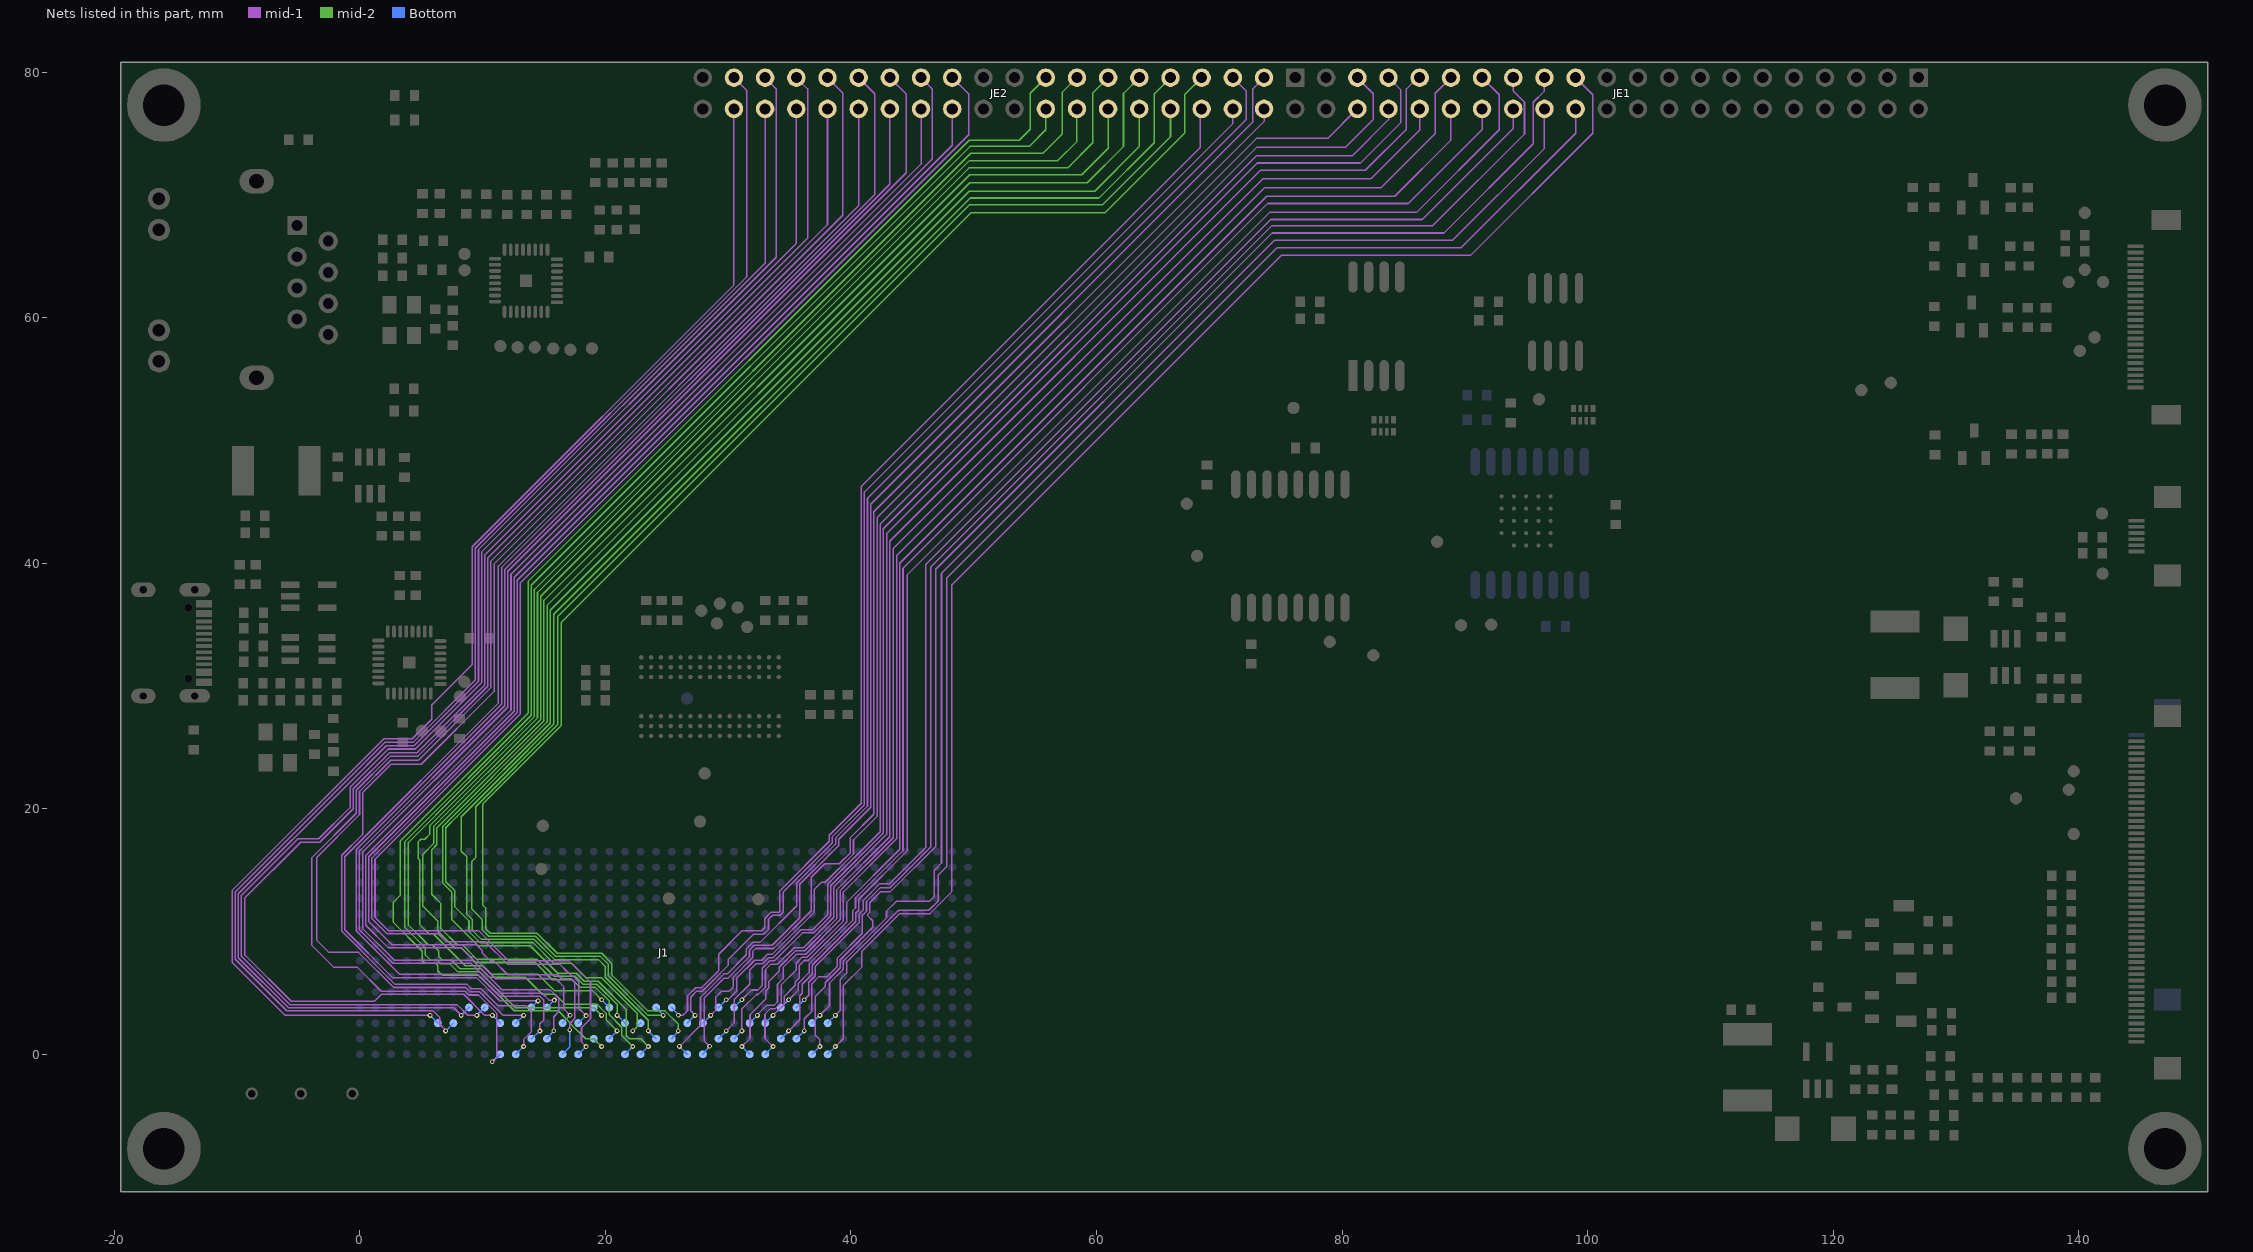
[diagram p0: the nets of this part, all layers, seen from the top]
# Altium PCB MISC105414.PcbDoc (part 5 of 11)
Units mm, origin at the board's own origin, x right, y up, seen from the top; angles counter-clockwise.
Board outline 170 x 92 mm, 6 copper layers (Top, GND, mid-1, mid-2, mid-3, Bottom), stack 1.231 mm thick; 238 components, 304 nets, 1456 pads, 1258 vias.
Unrouted connection lines stored in the file: 57.

## Via types
v1: diameter 0.4, hole 0.2, Top to Bottom, tented top, 618 vias
v2: diameter 0.5, hole 0.3, Top to Bottom, tented top, 522 vias
v3: diameter 0.5, hole 0.3, Top to Bottom, 41 vias
v4: diameter 1, hole 0.5, Top to Bottom, tented top, 36 vias
v5: diameter 0.7, hole 0.4, Top to Bottom, tented top, 34 vias
v6: diameter 1.3, hole 1.3, Top to Bottom, tented top, 3 vias
v7: diameter 4, hole 4, Top to Bottom, tented top, 2 vias
v8: diameter 3.3, hole 3.3, Top to Bottom, tented top, 2 vias

## Nets (pads, with @x,y where several pads share a name; then routed paths per layer and width w, separated by ;. In a path a pad name is that pad's centre, name@x,y a point inside that pad or via, vN(x,y) a via of type N, cw(c..) or ccw(c..) an arc to the next point about the centre after c; other vN are vias at no path point) (continued)
EXT_IO16: J1.Y10 JE1.23 | length 116.4
  mid-1 w0.127: v1(38.735,0.635) 39.37,1.27 39.37,5.594 40.896,7.12 40.896,8.39 43.97,11.465 46.438,11.465 48.2,13.227 48.2,38.2 75.1,65.1 90.5,65.1 100.421,75.021 100.421,78.159 JE1.23@99.03,79.55
  Bottom w0.127: J1.Y10@38.1,0 v1(38.735,0.635)
EXT_IO17: J1.A10 JE1.24 | length 109.9
  mid-1 w0.127: v1(38.735,3.175) 39.115,3.555 39.115,6.095 39.642,6.622 39.642,7.495 43.85,11.703 43.883,11.703 43.89,11.709 43.902,11.709 43.906,11.713 43.918,11.713 43.923,11.718 43.948,11.718 43.959,11.729 46.343,11.729 47.104,12.489 47.104,14.598 47.8,15.294 47.8,38.8 74.7,65.7 89.7,65.7 99.03,75.03 JE1.24@99.03,77.01
  Bottom w0.127: J1.A10@38.1,2.54 v1(38.735,3.175)
EXT_IO18: J1.Y11 JE1.25 | length 113.6
  mid-1 w0.127: v1(37.465,0.635) 37.465,1.195 37.102,1.558 37.102,4.717 37.913,5.528 37.913,5.82 39.134,7.04 39.134,7.707 41.771,10.345 41.771,10.879 41.353,11.297 41.353,11.387 41.522,11.556 41.522,12.343 42.429,13.251 43.217,13.251 46.9,16.934 46.9,39.5 74.3,66.9 88.3,66.9 95.576,74.176 95.576,77.556 96.49,78.469 JE1.25@96.49,79.55
  Bottom w0.127: J1.Y11@36.83,0 v1(37.465,0.635)
EXT_IO19: J1.A11 JE1.26 | length 109.3
  mid-1 w0.127: v1(37.465,3.175) 38.252,3.962 38.252,5.799 39.388,6.935 39.388,7.6 42.897,11.11 42.897,11.662 43.687,12.451 46.376,12.451 46.8,12.875 46.8,15 47.375,15.575 47.375,39.175 74.5,66.3 89,66.3 96.49,73.79 JE1.26@96.49,77.01
  Bottom w0.127: J1.A11@36.83,2.54 v1(37.465,3.175)
EXT_IO20: J1.Z12 JE1.27 | length 111.7
  mid-1 w0.127: v1(36.195,1.905) 36.195,2.885 36.821,3.511 36.821,5.754 37.399,6.332 38.066,6.332 38.868,7.134 38.868,7.801 40.918,9.851 40.918,11.312 41.267,11.66 41.267,12.448 42.369,13.55 43.157,13.55 46.5,16.893 46.5,39.7 74.3,67.5 87.4,67.5 94.863,74.963 94.863,77.556 93.95,78.469 JE1.27@93.95,79.55
  Bottom w0.127: J1.Z12@35.56,1.27 v1(36.195,1.905)
EXT_IO21: J1.B12 JE1.28 | length 105.1
  mid-1 w0.127: v1(36.195,4.445) 36.567,4.817 36.567,5.863 37.097,6.393 37.097,7.142 40.663,10.708 40.663,11.416 41.013,11.765 41.013,12.553 42.335,13.875 43.123,13.875 46.1,16.852 46.1,39.9 74.2,68 86.537,68 93.95,75.413 JE1.28@93.95,77.01
  Bottom w0.127: J1.B12@35.56,3.81 v1(36.195,4.445)
EXT_IO22: J1.Z13 JE1.29 | length 110.1
  mid-1 w0.127: v1(34.925,1.905) 35.832,2.812 35.832,4.77 36.029,4.967 36.029,5.712 36.842,6.526 36.842,7.246 40.396,10.8 40.396,11.508 40.627,11.739 40.627,12.628 44.6,16.601 44.6,39.073 74.127,68.6 86.1,68.6 92.8,75.3 92.8,78.16 JE1.29@91.41,79.55
  Bottom w0.127: J1.Z13@34.29,1.27 v1(34.925,1.905)
EXT_IO23: J1.B13 JE1.30 | length 103.6
  mid-1 w0.127: v1(34.925,4.445) 35.721,5.241 35.721,5.79 36.588,6.658 36.588,7.352 40.134,10.897 40.134,11.68 40.371,11.917 40.371,12.731 44.238,16.598 44.238,39.6 73.938,69.3 85.4,69.3 91.41,75.31 JE1.30@91.41,77.01
  Bottom w0.127: J1.B13@34.29,3.81 v1(34.925,4.445)
EXT_IO24: J1.Y14 JE1.31 | length 109.2
  mid-1 w0.127: v1(33.655,0.635) 33,1.29 33,3.275 33.45,3.725 33.846,3.725 34.308,4.187 34.308,5.642 35.538,6.872 35.538,7.416 36.019,7.897 36.415,7.897 39.384,10.865 39.384,13.228 43.714,17.558 43.714,40.6 73.714,70.6 83.2,70.6 87.6,75 87.6,78.28 JE1.31@88.87,79.55
  Bottom w0.127: J1.Y14@33.02,0 v1(33.655,0.635)
EXT_IO25: J1.A14 JE1.32 | length 103.9
  mid-1 w0.127: v1(33.655,3.175) 34.562,4.082 34.562,4.717 35.467,5.622 35.467,5.895 35.792,6.22 35.792,7.223 36.206,7.638 36.516,7.638 39.641,10.764 39.641,12.361 43.979,16.698 43.979,40 73.879,69.9 84.3,69.9 88.87,74.47 JE1.32@88.87,77.01
  Bottom w0.127: J1.A14@33.02,2.54 v1(33.655,3.175)
EXT_IO26: J1.Y15 JE1.33 | length 108.2
  mid-1 w0.127: v1(31.115,0.635) 31.775,1.295 31.775,3.225 33.05,4.5 33.05,5.135 33.292,5.377 33.292,5.916 34.15,6.775 34.15,7.097 35.485,8.432 36.232,8.432 38.857,11.057 38.857,13.42 43.159,17.722 43.159,41.8 73.359,72 81.9,72 85.25,75.35 85.25,78.634 86.167,79.55 JE1.33@86.33,79.55
  Bottom w0.127: v1(31.115,0.635) J1.Y15@31.75,0
EXT_IO27: J1.A15 JE1.34 | length 103
  mid-1 w0.127: v1(32.385,3.175) 32.385,3.235 33.129,3.979 33.741,3.979 34.018,4.257 34.018,5.712 34.475,6.169 34.475,7.063 35.566,8.154 36.313,8.154 39.116,10.957 39.116,13.319 43.439,17.642 43.439,41.2 73.539,71.3 82.35,71.3 86.33,75.28 JE1.34@86.33,77.01
  Bottom w0.127: J1.A15@31.75,2.54 v1(32.385,3.175)
EXT_IO28: J1.Z16 JE1.35 | length 107
  mid-1 w0.127: v1(31.115,1.905) 31.115,3.689 32.296,4.871 32.426,4.871 33.038,5.482 33.038,6.901 33.487,7.351 34.044,7.351 35.38,8.686 36.127,8.686 38.603,11.162 38.603,13.623 42.902,17.922 42.902,42.4 73.102,72.6 81.5,72.6 84.8,75.9 84.8,78.54 JE1.35@83.79,79.55
  Bottom w0.127: J1.Z16@30.48,1.27 v1(31.115,1.905)
EXT_IO29: J1.B16 JE1.36 | length 100.9
  mid-1 w0.127: v1(31.115,4.445) 31.908,5.238 32.422,5.238 32.784,5.599 32.784,7.007 33.382,7.606 33.761,7.606 36.044,9.888 36.97,9.888 38.349,11.267 38.349,13.738 42.638,18.027 42.638,42.8 73.038,73.2 80.85,73.2 83.79,76.14 JE1.36@83.79,77.01
  Bottom w0.127: J1.B16@30.48,3.81 v1(31.115,4.445)
EXT_IO30: J1.Z17 JE1.37 | length 106.2
  mid-1 w0.127: v1(29.845,1.905) 30.48,2.54 30.48,4.445 31.75,5.715 31.75,6.864 32.263,7.377 32.794,7.377 33.277,7.86 33.653,7.86 35.935,10.142 36.865,10.142 38.095,11.373 38.095,13.845 42.382,18.132 42.382,43.2 73.082,73.9 80.3,73.9 82.55,76.15 82.55,78.25 JE1.37@81.25,79.55
  Bottom w0.127: J1.Z17@29.21,1.27 v1(29.845,1.905)
EXT_IO31: J1.B17 JE1.38 | length 99
  mid-1 w0.127: v1(29.845,4.445) 29.99,4.445 30.683,5.138 30.683,6.188 32.162,7.668 32.726,7.668 33.191,8.132 33.566,8.132 37.022,11.589 37.022,13.433 37.609,14.021 37.912,14.021 40.208,16.317 40.208,17.458 42.127,19.377 42.127,43.697 73.031,74.6 78.84,74.6 JE1.38@81.25,77.01
  Bottom w0.127: J1.B17@29.21,3.81 v1(29.845,4.445)
EXT_IO32: J1.Y18 JE2.3 | length 99.9
  mid-1 w0.127: v1(28.483,0.651) 28.035,1.1 28.035,4.56 29.685,6.211 29.986,6.211 31.736,7.962 31.736,8.48 32.129,8.872 33.585,8.872 35.832,11.119 35.832,13.845 38.121,16.134 39.002,17.015 39.002,17.515 41.606,20.119 41.606,44.8 72.736,75.93 72.736,78.637 JE2.3@73.65,79.55
  Bottom w0.127: J1.Y18@27.94,0 v1(28.483,0.651)
EXT_IO33: J1.A18 JE2.4 | length 95.3
  mid-1 w0.127: v1(28.575,3.175) 29,3.6 29,4.675 29.443,5.118 30.055,5.118 30.396,5.459 30.396,6.262 31.99,7.857 31.99,8.374 32.234,8.618 33.693,8.618 36.768,11.694 36.768,14.422 37.858,15.512 39.043,15.512 39.954,16.422 39.954,17.654 41.861,19.561 41.861,44.2 73.65,75.989 JE2.4@73.65,77.01
  Bottom w0.127: J1.A18@27.94,2.54 v1(28.575,3.175)
EXT_IO34: J1.Y19 JE2.5 | length 99.9
  mid-1 w0.127: v1(26.027,0.643) 27.743,2.359 27.743,4.628 29.658,6.543 29.917,6.543 31.478,8.104 31.478,8.581 32.041,9.144 32.626,9.144 35.578,12.095 35.578,13.95 38.748,17.121 38.748,17.625 41.35,20.227 41.35,45.3 72.2,76.15 72.2,78.46 JE2.5@71.11,79.55
  Bottom w0.127: v1(26.027,0.643) J1.Y19@26.67,0
EXT_IO35: J1.A19 JE2.6 | length 94.3
  mid-1 w0.127: v1(27.305,3.175) 26.942,3.538 26.942,4.652 27.414,5.125 27.878,5.125 29.991,7.238 29.991,7.702 32.068,9.779 32.902,9.779 33.284,10.16 33.284,10.994 33.622,11.333 34.247,11.333 34.475,11.561 34.475,13.207 38.494,17.226 38.494,17.731 41.096,20.332 41.096,45.8 71.11,75.814 JE2.6@71.11,77.01
  Bottom w0.127: J1.A19@26.67,2.54 v1(27.305,3.175)
EXT_IO36: J1.Z20 JE2.7 | length 120.9
  mid-2 w0.127: v1(25.931,1.9) 25.931,2.459 24.859,3.53 23.464,3.53 20.503,6.492 20.503,7.422 19.7,8.225 16.075,8.225 14.434,9.866 10.609,9.866 10.239,10.236 10.239,11.92 10.006,12.153 10.006,20.382 16.4,26.776 16.4,35.18 49.77,68.55 60.7,68.55 67.2,75.05 67.2,78.18 JE2.7@68.57,79.55
  Bottom w0.127: J1.Z20@25.4,1.27 v1(25.931,1.9)
EXT_IO37: J1.B20 JE2.8 | length 94.1
  mid-1 w0.127: v1(25.949,3.179) 26.323,3.179 26.688,3.543 26.688,4.758 27.355,5.425 27.818,5.425 29.223,6.83 29.223,8.147 31.131,10.055 32.73,10.055 32.975,10.3 32.975,11.045 33.517,11.587 34.142,11.587 34.216,11.661 34.216,13.325 38.24,17.349 38.24,17.84 40.838,20.438 40.838,46.25 68.45,73.862 68.45,76.89 JE2.8@68.57,77.01
  Bottom w0.127: J1.B20@25.4,3.81 v1(25.949,3.179)
EXT_IO38: J1.Z21 JE2.9 | length 119.6
  mid-2 w0.127: 11.631,22.726 8.255,19.35 8.255,16.545 8.715,16.085 8.715,11.423 9.14,10.998 9.14,10.116 9.898,9.358 14.201,9.358 15.842,7.717 19.433,7.717 19.992,7.158 19.992,6.283 23.495,2.78 v1(23.495,1.905) ; 11.632,22.726 15.8,26.894 15.8,35.838 49.712,69.75 60.2,69.75 64.7,74.25 64.7,78.22 JE2.9@66.03,79.55
  Bottom w0.127: v1(23.495,1.905) J1.Z21@24.13,1.27
EXT_IO39: J1.B21 JE2.10 | length 116.2
  mid-2 w0.127: v1(24.709,3.167) 23.469,3.167 20.246,6.389 20.246,7.32 19.595,7.971 15.947,7.971 14.306,9.612 10.504,9.612 9.985,10.131 9.985,10.953 9.125,11.813 9.125,15.725 9.43,16.03 9.43,20.165 16.1,26.835 16.1,35.634 49.666,69.2 60.5,69.2 66.03,74.73 JE2.10@66.03,77.01
  Bottom w0.127: J1.B21@24.13,3.81 v1(24.709,3.167)
EXT_IO40: J1.Y22 JE2.11 | length 120.4
  mid-2 w0.127: v1(23.495,0.635) 22.874,1.256 21.963,1.256 21.705,1.514 21.705,3.657 19.409,5.954 18.27,5.954 17.617,6.607 16.118,6.607 13.875,8.85 9.613,8.85 7.484,10.979 7.484,13.213 6.74,13.958 6.74,18.554 15.247,27.061 15.247,36.566 49.682,71 59.25,71 62.2,73.95 62.2,78.26 JE2.11@63.49,79.55
  Bottom w0.127: J1.Y22@22.86,0 v1(23.495,0.635)
EXT_IO41: J1.A22 JE2.12 | length 116.1
  mid-2 w0.127: v1(22.225,1.905) 22.589,2.269 22.589,3.326 19.691,6.223 18.439,6.223 17.262,7.4 15.8,7.4 14.096,9.104 9.793,9.104 8.886,10.011 8.886,10.856 7.738,12.003 7.738,13.318 6.994,14.063 6.994,18.448 7.915,19.369 15.503,26.957 15.503,36.166 49.637,70.3 59.85,70.3 63.49,73.94 JE2.12@63.49,77.01
  Bottom w0.127: v1(22.225,1.905) J1.A22@22.86,2.54
EXT_IO42: J1.Y23 JE2.13 | length 119.5
  mid-2 w0.127: v1(22.225,0.635) 21.331,1.529 21.331,2.209 20.305,3.235 20.305,4.339 19.198,5.446 17.947,5.446 17.315,6.078 15.672,6.078 14.276,7.474 9.44,7.474 8.25,8.664 7.736,8.664 6.35,10.05 6.35,10.85 5.137,12.063 5.137,16.296 6.006,17.165 6.006,18.546 14.733,27.273 14.733,37.316 49.618,72.2 57.65,72.2 59.7,74.25 59.7,78.3 JE2.13@60.95,79.55
  Bottom w0.127: J1.Y23@21.59,0 v1(22.225,0.635)
EXT_IO43: J1.A23 JE2.14 | length 113.9
  mid-2 w0.127: v1(20.955,3.175) 20.955,4.048 19.303,5.7 18.165,5.7 17.511,6.353 15.822,6.353 14.447,7.728 9.545,7.728 8.356,8.918 7.932,8.918 6.604,10.246 6.604,12.291 5.85,13.045 5.85,16.649 6.261,17.06 6.261,18.437 14.988,27.163 14.988,36.966 49.672,71.65 58.8,71.65 60.95,73.8 JE2.14@60.95,77.01
  Bottom w0.127: v1(20.955,3.175) J1.A23@21.59,2.54
EXT_IO44: J1.Z24 JE2.15 | length 117.1
  mid-2 w0.127: v1(20.955,1.905) 20.051,2.809 20.051,3.324 19.309,4.067 16.709,4.067 15.878,4.898 14.85,4.898 13.477,6.271 10.562,6.271 9.867,6.966 8.159,6.966 7.475,7.65 6.725,7.65 6.438,7.937 6.438,8.384 5.904,8.918 5.56,8.918 3.95,10.527 3.95,17.25 8.361,21.661 14.214,27.514 14.214,37.866 49.749,73.4 55.65,73.4 57.2,74.95 57.2,78.34 JE2.15@58.41,79.55
  Bottom w0.127: J1.Z24@20.32,1.27 v1(20.955,1.905)
EXT_IO45: J1.B24 JE2.16 | length 111.4
  mid-2 w0.127: v1(19.685,4.445) 18.938,5.192 15.833,5.192 14.5,6.525 10.704,6.525 10.009,7.22 8.58,7.22 5.98,9.82 5.62,9.82 4.864,10.575 4.864,15.838 4.737,15.966 4.737,17.301 4.949,17.513 5.278,17.513 5.703,17.939 5.703,18.638 14.469,27.403 14.469,37.616 49.653,72.8 56.85,72.8 58.41,74.36 JE2.16@58.41,77.01
  Bottom w0.127: v1(19.685,4.445) J1.B24@20.32,3.81
EXT_IO46: J1.Z25 JE2.17 | length 116
  mid-2 w0.127: v1(19.685,0.635) 19.05,1.27 18.391,1.27 17.145,2.516 17.145,2.549 16.155,3.539 12.575,3.539 9.881,6.232 9.843,6.232 9.617,6.458 6.692,6.458 6.35,6.8 6.35,7.223 6.151,7.421 5.279,7.421 5.075,7.625 5.075,8.4 2.7,10.775 2.7,12.35 3.275,12.925 3.275,17.353 13.7,27.778 13.7,38.516 49.634,74.45 53.7,74.45 54.6,75.35 54.6,78.28 JE2.17@55.87,79.55
  Bottom w0.127: J1.Z25@19.05,1.27 v1(19.685,0.635)
EXT_IO47: J1.B25 JE2.18 | length 111.4
  mid-2 w0.127: v1(19.685,3.175) 19.067,3.793 12.68,3.793 9.76,6.712 7.988,6.712 7.337,7.363 6.587,7.363 6.275,7.675 5.75,7.675 5.336,8.089 5.336,8.664 3.639,10.361 3.639,17.298 13.96,27.619 13.96,38.216 49.694,73.95 54.515,73.95 55.87,75.305 JE2.18@55.87,77.01
  Bottom w0.127: J1.B25@19.05,3.81 v1(19.685,3.175)
EXT_IO48: J1.Y26 JE2.23 | length 115.3
  mid-1 w0.127: v1(18.431,0.629) 18.052,1.008 18.052,2.16 18.787,2.896 18.787,5.857 17.04,7.604 12.128,7.604 9.658,10.075 2.313,10.075 1.233,11.154 1.233,15.887 13.05,27.704 13.077,27.704 13.077,38.4 49.588,74.911 49.588,78.212 JE2.23@48.25,79.55
  Bottom w0.127: J1.Y26@17.78,0 v1(18.431,0.629)
EXT_IO49: J1.A26 JE2.24 | length 108.4
  mid-1 w0.127: v1(18.423,3.151) 17.825,3.749 17.825,5.908 17.325,6.408 17.208,6.408 16.885,6.731 16.267,7.349 12.018,7.349 10.196,9.172 7.021,9.172 6.373,9.82 2.208,9.82 0.979,11.049 0.979,15.992 12.822,27.835 12.822,38.622 48.25,74.05 JE2.24@48.25,77.01
  Bottom w0.127: J1.A26@17.78,2.54 v1(18.423,3.151)
EXT_IO50: J1.Y27 JE2.25 | length 113.4
  mid-1 w0.127: v1(17.096,1.99) 17.096,2.498 17.508,2.91 17.508,5.866 17.22,6.154 16.445,6.154 16.123,6.477 12.052,6.477 10.931,7.598 10.633,7.598 9.957,8.275 9.957,8.474 9.513,8.918 2.617,8.918 0.725,10.809 0.725,16.097 12.567,27.939 12.567,38.867 46.623,72.923 46.623,78.637 JE2.25@45.71,79.55
  Bottom w0.127: J1.Y27@16.51,0 17.096,0.586 v1(17.096,1.99)
EXT_IO51: J1.A27 JE2.26 | length 106.9
  mid-1 w0.127: v1(17.121,3.181) 16.62,3.682 16.62,5.484 15.95,6.154 11.075,6.154 9.3,7.929 9.024,7.929 8.29,8.664 2.326,8.664 0.471,10.518 0.471,16.203 12.309,28.041 12.309,39.109 45.71,72.51 JE2.26@45.71,77.01
  Bottom w0.127: J1.A27@16.51,2.54 v1(17.121,3.181)
EXT_IO52: J1.Z28 JE2.27 | length 110.2
  mid-1 w0.127: v1(15.791,1.914) 15.791,3.065 16.204,3.478 16.204,4.565 15.524,5.246 11.587,5.246 9.157,7.675 2.793,7.675 0.217,10.251 0.217,16.457 11.998,28.237 12.053,28.237 12.053,39.353 44.503,71.803 44.503,78.217 JE2.27@43.17,79.55
  Bottom w0.127: J1.Z28@15.24,1.27 v1(15.791,1.914)
EXT_IO53: J1.B28 JE2.28 | length 103.9
  mid-1 w0.127: v1(15.841,4.415) 15.405,4.415 14.846,4.974 11.499,4.974 9.051,7.421 2.688,7.421 -0.037,10.146 -0.037,16.562 11.799,28.397 11.799,39.499 43.17,70.87 JE2.28@43.17,77.01
  Bottom w0.127: J1.B28@15.24,3.81 v1(15.841,4.415)
EXT_IO54: J1.Z29 JE2.29 | length 108.7
  mid-1 w0.127: v1(14.658,1.896) 14.658,2.487 14.968,2.797 14.968,4.42 14.669,4.719 11.394,4.719 9.605,6.508 3.242,6.508 -0.291,10.041 -0.291,16.674 11.544,28.509 11.544,39.644 41.939,70.039 41.939,78.241 JE2.29@40.63,79.55
  Bottom w0.127: J1.Z29@13.97,1.27 v1(14.658,1.896)
EXT_IO55: J1.B29 JE2.30 | length 103.1
  mid-1 w0.127: v1(14.519,4.356) 11.398,4.356 9.502,6.252 2.662,6.252 -1.225,10.139 -1.225,16.1 11.283,28.608 11.283,39.783 40.63,69.13 JE2.30@40.63,77.01
  Bottom w0.127: J1.B29@13.97,3.81 v1(14.519,4.356)
EXT_IO56: J1.Y30 JE2.31 | length 110.6
  mid-1 w0.127: v1(13.335,0.635) 13.335,1.195 13.974,1.834 13.974,3.539 13.562,3.95 11.252,3.95 9.866,5.337 9.081,5.337 8.724,5.694 2.861,5.694 -1.479,10.034 -1.479,16.205 0.221,17.904 0.221,21.304 2.536,23.619 4.999,23.619 10.931,29.551 10.931,39.931 39.334,68.334 39.334,78.306 JE2.31@38.09,79.55
  Bottom w0.127: J1.Y30@12.7,0 v1(13.335,0.635)
EXT_IO57: J1.A30 JE2.32 | length 106.6
  mid-1 w0.127: v1(13.343,3.168) 11.67,3.168 11.412,3.425 11.412,3.431 9.761,5.083 8.975,5.083 8.617,5.44 2.756,5.44 -0.104,8.3 -2.525,8.3 -3.5,9.275 -3.5,16.058 -0.033,19.525 -0.033,21.409 2.515,23.957 4.765,23.957 10.677,29.87 10.677,40.177 38.09,67.59 JE2.32@38.09,77.01
  Bottom w0.127: J1.A30@12.7,2.54 v1(13.343,3.168)
EXT_IO58: J1.Y31 JE2.33 | length 111.5
  mid-1 w0.127: v1(10.785,-0.607) 11.158,-0.233 11.158,3.326 9.655,4.829 8.866,4.829 8.557,5.137 1.75,5.137 -0.188,7.075 -2.112,7.075 -3.937,8.9 -3.937,15.98 -0.287,19.63 -0.287,21.515 2.489,24.291 4.735,24.291 10.423,29.979 10.423,40.423 36.463,66.463 36.463,78.637 JE2.33@35.55,79.55
  Bottom w0.127: v1(10.785,-0.607) J1.Y31@11.43,0
EXT_IO59: J1.A31 JE2.34 | length 113.3
  mid-1 w0.127: v1(10.795,3.175) 10.16,3.175 8.452,4.883 1.762,4.883 1.191,4.311 -5.581,4.311 -9.313,8.043 -9.321,8.043 -9.396,8.117 -9.396,12.702 -4.826,17.272 -3.265,17.272 -0.541,19.996 -0.541,21.62 2.384,24.545 4.628,24.545 10.169,30.086 10.169,40.669 35.55,66.05 JE2.34@35.55,77.01
  Bottom w0.127: v1(10.795,3.175) J1.A31@11.43,2.54
EXT_IO60: J1.B32 JE2.35 | length 114.4
  mid-1 w0.127: v1(9.525,3.175) 8.778,3.175 7.906,4.047 -5.719,4.047 -9.65,7.977 -9.65,12.954 -5.049,17.555 -3.341,17.555 -0.795,20.101 -0.795,21.761 2.312,24.868 4.512,24.868 9.915,30.272 9.915,40.915 33.923,64.923 33.923,78.637 JE2.35@33.01,79.55
  Bottom w0.127: v1(9.525,3.175) J1.B32@10.16,3.81
EXT_IO61: J1.B33 JE2.36 | length 109.2
  mid-1 w0.127: v1(8.255,3.175) 7.637,3.793 -5.825,3.793 -9.904,7.872 -9.904,13.073 -1.058,21.919 2.146,25.122 4.406,25.122 9.661,30.377 9.661,32.636 ; 9.66,32.637 9.66,41.109 33.01,64.458 JE2.36@33.01,77.01
  Bottom w0.127: v1(8.255,3.175) J1.B33@8.89,3.81
EXT_IO62: J1.A34 JE2.37 | length 111.7
  mid-1 w0.127: v1(6.985,1.905) 7.013,1.933 6.504,2.442 6.504,2.996 5.961,3.538 -5.951,3.538 -10.158,7.745 -10.158,13.221 2.056,25.434 4.359,25.434 9.404,30.48 9.404,41.217 31.5,63.313 31.5,78.52 JE2.37@30.47,79.55
  Bottom w0.127: v1(6.985,1.905) J1.A34@7.62,2.54
EXT_IO63: J1.A35 JE2.38 | length 106.6
  mid-1 w0.127: v1(5.715,3.175) -6.096,3.175 -10.414,7.493 -10.414,13.332 1.963,25.709 4.274,25.709 5.853,27.288 5.853,28.453 9.146,31.746 9.146,41.332 30.47,62.656 JE2.38@30.47,77.01
  Bottom w0.127: v1(5.715,3.175) J1.A35@6.35,2.54